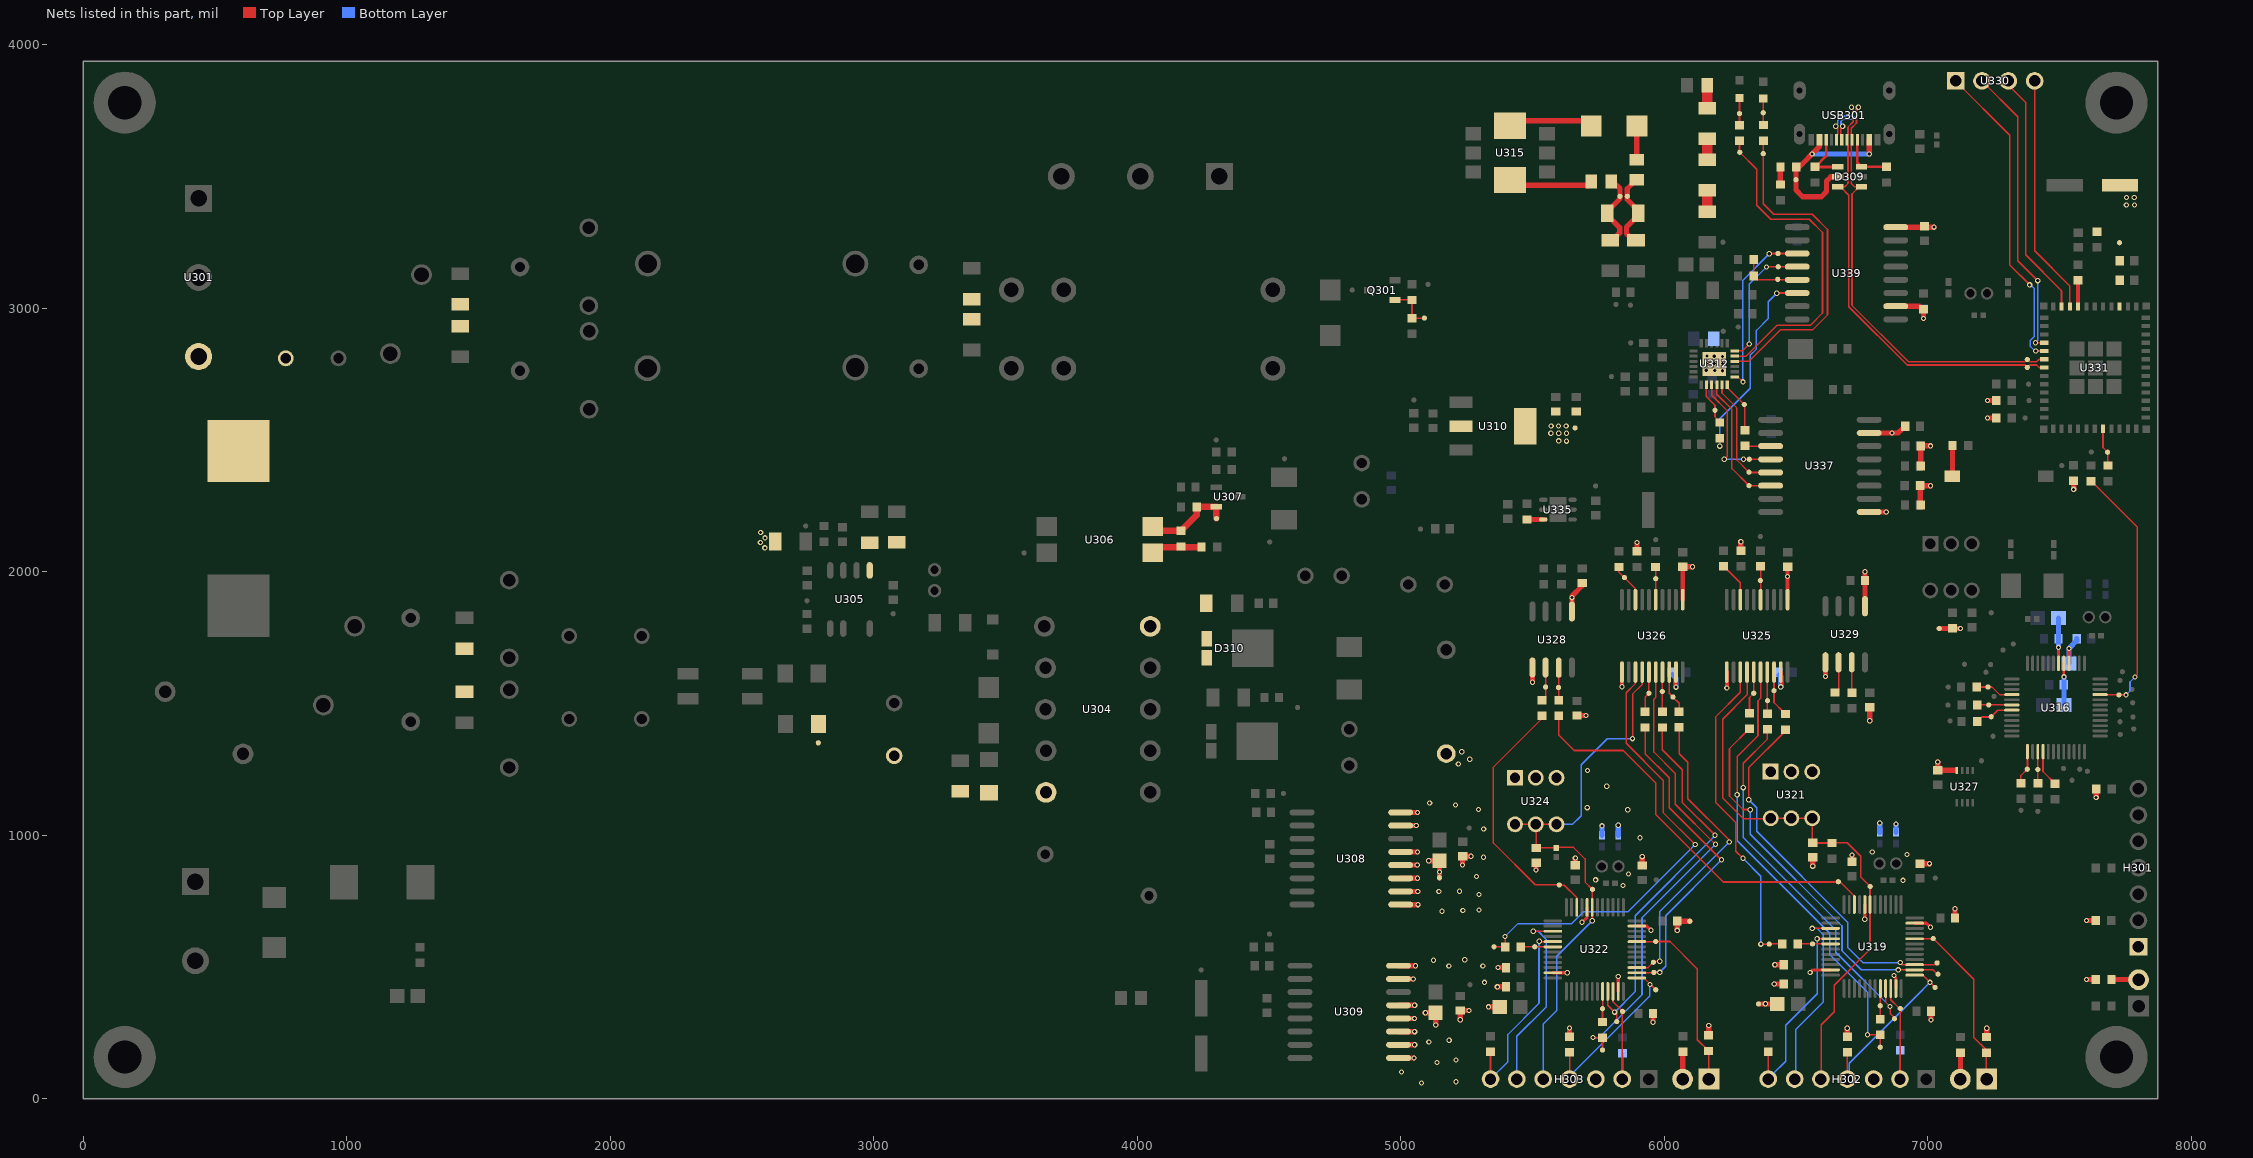
[diagram p0: the nets of this part, all layers, seen from the top]
# Altium PCB MISC84429.PcbDoc (part 4 of 5)
Units mil, origin at the board's own origin, x right, y up, seen from the top; angles counter-clockwise.
Board outline 7874.02 x 3937.01 mil, 4 copper layers (Top Layer, GND, POWER, Bottom Layer); 424 components, 202 nets, 1144 pads, 784 vias.

## Via types
v1: diameter 20, hole 12, Top Layer to Bottom Layer, tented both sides, 695 vias
v2: diameter 20, hole 12, Top Layer to Bottom Layer, 87 vias
v3: diameter 30, hole 15, Top Layer to Bottom Layer, tented both sides, 2 vias

## Nets (pads, with @x,y where several pads share a name; then routed paths per layer and width w, separated by ;. In a path a pad name is that pad's centre, name@x,y a point inside that pad or via, vN(x,y) a via of type N, cw(c..) or ccw(c..) an arc to the next point about the centre after c; other vN are vias at no path point) (continued)
NetD308_1: D308.1 L309.2 | length 97.4
  Top Layer w20: L309.2@5896,3563.04 5896,3659 D308.1@5897,3660
NetD308_2: D308.2 U315.8 | length 299.9
  Top Layer w20: U315.8@5415.01,3691.96 U315.8@5439.06,3716 ; U315.8@5440.06,3711 D308.2@5706,3711
NetD309_3: D309.3 R406.2 USB301.4 | length 203.4
  Top Layer w10: USB301.4@6733.21,3638.49 6733.21,3551.44 6748.98,3535.66 R406.2@6843,3535.66
NetD309_4: D309.4 R408.2 USB301.10 | length 205.2
  Top Layer w10: USB301.10@6615.1,3638.49 6615.1,3577.1 6573.66,3535.66 6573.92,3535.4 D309.4@6658.76,3535.4
NetD309_5: D309.5 R405.2 TP427.1 USB301.2 USB301.11 | length 723
  Top Layer w20: USB301.11@6589.51,3638.49 6589.51,3612.51 6500,3523 TP427.1@6500,3487 6500,3448 6526,3422 6596,3422 6616,3442 6616,3482 6632,3498 D309.5@6658.76,3498 ; v1(6778.49,3584.49) USB301.2@6778.49,3638.49
  Bottom Layer w20: v1(6561.51,3584.49) v1(6778.49,3584.49)
NetD310_1: D310.1 D310.2 R432.1 U304.10
NetF301_1: F301.1 F302.1 U301.3
NetL307_1: L307.1 U312.25
  other v1: 6222,2762 6192,2763 6160,2764 6221,2789 6160,2790 6191,2790 6221,2816 6190,2817 6162,2818
NetL308_2: L308.2 R339.2 | length 70.8
  Top Layer w40: R339.2@6163,3758.22 L308.2@6163,3829
NetL309_1: L309.1 R342.1 R344.2 TP341.1 | length 271.9
  Top Layer w20: R344.2@5877,3263 5857,3283 5857,3307 5901.22,3351.22 R342.1@5901.22,3360 5901.22,3370.78 5860,3412 5860,3453 L309.1@5887,3480
NetL310_1: L310.1 R338.2 R342.2 TP339.1 | length 287.9
  Top Layer w20: R342.2@5793.5,3377.5 5784.78,3368.78 R342.2@5784.78,3360 5784.78,3352.22 5831,3306 5831,3285 R338.2@5808,3262 ; R342.2@5794,3377 5832,3415 5832,3454 L310.1@5805,3481 ; R338.2@5796,3257.22 R338.2@5805.22,3257.22
NetL310_2: L310.2 U315.7 | length 311.6
  Top Layer w20: U315.7@5415.01,3486.04 U315.7@5438.06,3463 ; U315.7@5438.06,3466 L310.2@5710,3466 ; L310.2@5710,3463 L310.2@5715,3468
NetQ301_1: Q301.1 R306.2 R307.1 TP302.1 | length 164.2
  Top Layer w6: Q301.1@4990,3031 5040,3031 5043,3028 R306.2@5043,2961.66 TP302.1@5086.66,2961.66
NetR301_1: R301.1 R304.2
NetR303_1: R303.1 R305.2
NetR308_1: R308.1 R311.2
NetR315_1: R315.1 R316.2 U306.1 | length 157.3
  Top Layer w25: U306.1@4087,2093 R315.1@4244.34,2093
NetR316_1: R316.1 R322.1 TP311.1 U306.2 U307.2 | length 297.9
  Top Layer w25: U306.2@4087.66,2154.66 R316.1@4166,2154.66 4226,2214.66 4226,2242 R322.1@4225,2243 ; R322.1@4236.4,2245.4 U307.2@4300.31,2245.4 TP311.1@4300.31,2203.31
NetR319_2: R319.2 R320.2 U305.5
NetR328_1: R328.1 TP320.1 U312.24 | length 202.5
  Top Layer w6: U312.24@6239.21,2699.79 U312.24@6239.21,2709.33 6239.21,2698.79 6306,2632 R328.1@6306,2544
NetR330_1: R330.1 TP324.1 U312.20 | length 157
  Top Layer w6: U312.20@6160.47,2709.33 6160.47,2663.53 6193,2631 TP324.1@6193,2612 6193,2587 R330.1@6208,2572
NetR334_1: R334.1 TP327.1 U313.2 | length 100.3
  Top Layer w6: R334.1@6376.74,3694.64 U313.2@6376.74,3794.92
NetR334_2: R334.2 TP329.1 U312.4 | length 1279.7
  Top Layer w6: U312.4@6268.4,2797.85 6321.85,2797.85 6441,2917 6563,2917 6620,2974 6620,3298 6562,3356 6416,3356 6376,3396 TP329.1@6376,3586 ; 6376.74,3600.26 6376.74,3609 ; R334.2@6376.74,3635.32 6376.74,3609 ; TP329.1@6378,3588 6376.74,3589.26 6376.74,3609
NetR335_1: R335.1 TP328.1 U314.1 | length 103.8
  Top Layer w6: R335.1@6286,3693.66 TP328.1@6286,3738 U314.1@6286,3797.5
NetR335_2: R335.2 TP330.1 U312.5 | length 1270.2
  Top Layer w6: U312.5@6268.4,2817.53 6310.53,2817.53 6428,2935 6555,2935 6601,2981 6601,3287 6551,3337 6404,3337 6351,3390 6351,3527 6286,3592 R335.2@6286,3634.34
NetR339_1: R339.1 R340.1 | length 65.8
  Top Layer w40: R340.1@6163,3563.22 R339.1@6163,3629
NetR340_2: R340.2 R341.2 | length 75.8
  Top Layer w40: R341.2@6163,3366.22 R340.2@6163,3442
NetR346_2: R346.2 TP346.1 U316.45 | length 999.7
  Top Layer w6: R346.2@7620,2343.34 R346.2@7630.67,2332.67 ; R346.2@7631,2333 7796,2168 7796,1609 v1(7787,1600) ; U316.45@7654.32,1533.21 TP346.1@7724.79,1533.21 ; TP346.1@7726,1532 v1(7753,1532)
  Bottom Layer w6: v1(7753,1532) 7768,1547 7768,1581 v1(7787,1600)
NetR348_1: R348.1 TP366.1 U316.16 | length 145.9
  Top Layer w6: R348.1@7185.66,1562 TP366.1@7229,1562 7244,1562 7272.79,1533.21 U316.16@7319.68,1533.21
NetR349_1: R349.1 TP368.1 U316.18 | length 131.4
  Top Layer w6: R349.1@7188.66,1493 7189.5,1493.84 U316.18@7319.68,1493.84
NetR350_1: R350.1 TP370.1 U316.19 | length 149.9
  Top Layer w6: R350.1@7187.66,1431 7204.66,1448 7240,1448 TP370.1@7241,1449 7266.16,1474.16 U316.19@7319.68,1474.16
NetR351_2: R351.2 U316.28 | length 141.2
  Top Layer w6: U316.28@7437.79,1316.68 7437.79,1240.87 R351.2@7484,1194.66
NetR352_2: R352.2 TP372.1 U316.27 | length 119.9
  Top Layer w6: R352.2@7418.1,1196.76 U316.27@7418.1,1316.68
NetR353_2: R353.2 TP375.1 U316.25 | length 130.3
  Top Layer w6: R353.2@7354,1196.66 7354,1226 TP375.1@7378,1250 7378.73,1250.73 U316.25@7378.73,1316.68
NetR355_1: R355.1 U317.2 | length 90.3
  Top Layer w20: R355.1@7697.66,452 U317.2@7788,452
NetR361_1: R361.1 TP382.1 U319.18 | length 118.7
  Top Layer w6: R361.1@6512.84,586.84 U319.18@6631.55,586.84
NetR362_1: R362.1 U320.2 | length 65
  Top Layer w20: U320.2@7125,109 R362.1@7125,174
NetR364_2: R364.2 TP384.1 U319.32 | length 112
  Top Layer w6: R364.2@6820.53,305.53 U319.32@6820.53,417.55
NetR370_1: R370.1 U323.2 | length 102.1
  Top Layer w20: U323.2@6071,75.22 R370.1@6071,177.34
NetR372_1: R372.1 TP395.1 U322.18 | length 121.7
  Top Layer w6: R372.1@5455.66,576 TP395.1@5509,576 ; TP395.1@5509.16,575.84 U322.18@5577.55,575.84
NetR373_2: R373.2 TP397.1 U322.32 | length 116.1
  Top Layer w6: R373.2@5766,290.66 TP397.1@5766,341 5766.53,341.53 U322.32@5766.53,406.55
NetR378_2: R378.2 TP406.1 U325.18 | length 165.1
  Top Layer w6: U325.18@6416.98,1618.56 6416.98,1503.02 R378.2@6452,1468
NetR379_1: R379.1 TP408.1 U325.5 | length 127.2
  Top Layer w6: R379.1@6365,2020.34 6365.79,2019.55 U325.5@6365.79,1893.44
NetR380_2: R380.2 TP409.1 U325.17 | length 154.2
  Top Layer w6: R380.2@6391.39,1464.39 U325.17@6391.39,1618.56
NetR381_2: R381.2 TP410.1 U325.15 | length 158.2
  Top Layer w6: R381.2@6324,1472 6324,1522 TP410.1@6340,1538 ; R381.2@6328,1467 R381.2@6328,1472 ; TP410.1@6340.2,1538 U325.15@6340.2,1618.56
NetR382_1: R382.1 U325.8 | length 153
  Top Layer w6: R382.1@6226,2020.34 6289.02,1957.32 U325.8@6289.02,1893.44
NetR383_1: R383.1 TP413.1 U326.5 | length 124
  Top Layer w6: U326.5@5967.79,1893.44 5967.79,2017.13 R383.1@5968,2017.34
NetR384_2: R384.2 TP411.1 U326.18 | length 165.6
  Top Layer w6: U326.18@6018.98,1618.56 6018.98,1538.02 TP411.1@6033,1524 6057,1500 R384.2@6057,1468.66
NetR385_2: R385.2 TP414.1 U326.17 | length 151.1
  Top Layer w6: R385.2@5993,1467.66 5993.39,1468.05 U326.17@5993.39,1618.56
NetR386_2: R386.2 TP415.1 U326.15 | length 156.8
  Top Layer w6: R386.2@5928,1467.66 5928,1524 TP415.1@5942,1538 5942.2,1538.2 U326.15@5942.2,1618.56
NetR387_1: R387.1 TP416.1 U326.8 | length 150
  Top Layer w6: R387.1@5828,2017.34 5828,1998 5891.02,1934.98 U326.8@5891.02,1893.44
NetR388_2: R388.2 TP417.1 U328.7 | length 123.8
  Top Layer w6: R388.2@5600,1511.66 U328.7@5600,1635.5
NetR389_2: R389.2 TP418.1 U328.6 | length 109.8
  Top Layer w6: R389.2@5550,1525.66 U328.6@5550,1635.5
NetR393_2: R393.2 U329.7 | length 113.5
  Top Layer w6: R393.2@6712,1542 U329.7@6712,1655.5
NetR395_2: R395.2 U329.6 | length 102.5
  Top Layer w6: R395.2@6662,1553 U329.6@6662,1655.5
NetR401_2: R401.2 U331.8 | length 95.7
  Top Layer w15: U331.8@7571.02,3006.29 R401.2@7571.02,3102.02
NetR403_2: R403.2 TP425.1 U331.31 | length 146.7
  Top Layer w6: U331.31@7665.51,2541.72 7665.51,2470.49 TP425.1@7683,2453 7684,2452 R403.2@7684,2402.66
NetR404_1: R404.1 R405.1 | length 66
  Top Layer w20: R404.1@6441,3468.66 R405.1@6441,3534.66
NetR407_2: R407.2 SW301.1 | length 109.2
  Top Layer w20: SW301.1@7093.83,2362 R407.2@7093.83,2471.17
NetR416_2: R416.2 U335.6 | length 52
  Top Layer w20: R416.2@5489.6,2197.6 U335.6@5541.59,2197.6
PGND: C324.2 C325.1 C328.2 C330.2 C331.1 C369.1 C370.2 C371.2 C372.2 C373.2 C374.2 C375.1 C376.1 C377.2 C378.1 C379.1 C380.2 C381.2 C382.2 C383.2 C384.2 C385.1 C386.1 C387.2 C388.1 C390.2 C392.2 C395.2 C397.2 H302.3 H303.3 R363.2 R368.2 R371.1 R377.2 TP403.1 TP404.1 TP405.1 U308.9 U308.10 U308.11 U308.12 U308.13 U308.15 U308.16 U309.9 U309.10 U309.11 U309.12 U309.13 U309.15 U309.16 U319.8 U319.23 U319.35 U319.47 U321.1 U321.2 U321.3 U322.8 U322.23 U322.35 U322.47 U324.1 U324.2 U324.3 U325.11 U325.19 U326.11 U326.19 U328.5 U329.5 | length 3086.6
  Top Layer w12: U322.23@5577.55,477.42 v1(5632.42,477.42) ; v1(5688,669) 5707.47,688.47 U322.8@5707.47,725.45 ; U322.35@5825.58,406.55 v1(5825.58,463.58) ; U322.47@5896.45,654.58 5934.42,654.58 v1(5950,639) ; v1(6554,478) 6564.42,488.42 U319.23@6631.55,488.42 ; v1(6761.47,680.47) U319.8@6761.47,736.45 ; v1(6872,467) 6871,466 6879.58,457.42 U319.35@6879.58,417.55 ; U319.47@6950.45,665.58 6995.42,665.58 v1(7011,650)
  Top Layer w15: v1(5839.84,1562.84) U326.11@5839.84,1618.56 ; v1(6044.57,1561.43) U326.19@6044.57,1618.56 ; v1(6237.84,1557.84) U325.11@6237.84,1618.56 ; v1(6442.57,1562.43) U325.19@6442.57,1618.56
  Top Layer w20: U309.9@4992.02,154 v1(5051,154) ; U309.10@4992.02,204 v1(5053,204) ; U309.11@4992.02,254 v1(5053,254) ; U309.12@4992.02,304 v1(5052,304) ; U309.13@4992.02,354 v1(5053,354) ; U309.15@4992.02,454 v1@5047,454 ; U309.16@4992.02,504 v1(5056,504) ; U308.9@5000.02,736 v1(5066,736) ; U308.10@5000.02,786 v1(5065,786) ; U308.11@5000.02,836 v1(5064,836) ; U308.12@5000.02,886 v1(5063,886) ; U308.13@5000.02,936 v1(5064,936) ; U308.15@5000.02,1036 v1(5059,1036) ; U308.16@5000.02,1086 v1(5064,1086) ; v1(5093.63,325.63) C331.1@5133,325.63 v1(5133,279) ; v1(5106.63,902.63) C325.1@5147,902.63 v1(5147,860) TP403.1@5147,838 ; v1(5226,299) C330.2@5226,334.44 v1(5259.44,334.44) ; v1(5235,886) C324.2@5235,919.44 v1(5266.56,919.44) ; v1(5333,348) C385.1@5375.63,348 ; v1(5367,424) C386.1@5399.44,424 ; v1(5369,497) C387.2@5399.44,497 ; v1(5500,1580) U328.5@5500,1635.5 ; v1(5514,867) C388.1@5514,895.44 ; R377.2@5641,234.66 v1(5641,268) ; C381.2@5663,885.56 v1(5663,913) ; C395.2@5669,1453.44 v1(5703.44,1453.44) ; C382.2@5917,884.56 v1(5917,918) ; v1(5957.56,289.56) C384.2@5957.56,323 ; v1(6049.56,638.44) C383.2@6049.56,674 ; C383.2@6057,673 TP404.1@6097,673 ; R371.1@6169,239.66 v1(6169,277) ; TP405.1@6358,359 v1@6384,359 ; v1(6384,360) v1@6384,359 ; v1(6418,435) C376.1@6453.44,435 ; v1(6420,508) C377.2@6453.44,508 ; C375.1@6422,359 v1@6384,359 ; v1(6564,882) C378.1@6564,915.44 ; v1(6612,1602) U329.5@6612,1655.5 ; R368.2@6695,234.66 v1(6695,267) ; C371.2@6713,898.56 v1(6713,924) ; v1(6780,1434) C397.2@6780,1485.44 ; C372.2@6971,891.56 v1(7006.56,891.56) ; v1(7012.56,298.56) C374.2@7012.56,331 ; C373.2@7103.56,685 v1(7103.56,720.56) ; R363.2@7224,233.66 v1(7224,267)
  Bottom Layer w20: C379.1@5764,999.46 v1(5764,1035) ; C380.2@5826,999.46 v1(5826,1037) ; C392.2@6032,1609 6044.57,1596.43 v1(6044.57,1561.43) ; C390.2@6436,1607 6442.57,1600.43 v1(6442.57,1562.43) ; C369.1@6818,1010.46 v1(6818,1046) ; C370.2@6880,1010.46 v1(6880,1042)
  other v1: 5079,59 5210,64 5003,101 5138,137 5210,146 5107,215 5184,221 5318,441 5048,454 5183,503 5312,503 5125,525 5243,527 5157,711 5236,714 5297,716 5297,774 5145,786 5223,787 5844,809 6906,828 5740,830 5288,843 5865,852 5314,916 6922,926 6790,936 5908,990 5315,1023 5862,1096 5295,1097 5708,1104 5208,1114 5110,1122 5782,1185 5709,1245
  other v2: 5219,1270 5262,1288 5232,1316
STPM32_CS: TP323.1 U312.21 U337.12 | length 484.1
  Top Layer w6: U312.21@6180.16,2709.33 6180.16,2668.84 6240,2609 6240,2438 v2(6228,2426) ; v2(6301,2426) TP323.1@6323,2426 ; TP323.1@6328,2426 U337.12@6403.98,2426
  Bottom Layer w6: v2(6228,2426) v2(6301,2426)
STPM32_EN: R336.1 R337.2 TP337.1 U339.5 | length 228.2
  Top Layer w6: R337.2@6339.66,3123.34 R336.1@6339.66,3184 ; R337.2@6342,3118 6353,3107 U339.5@6504.98,3107
STPM32_INT1: TP332.1 U312.6 U339.4 | length 473.6
  Top Layer w6: U312.6@6268.4,2837.22 6296.22,2837.22 v2(6323,2864) ; v2(6388,3156) U339.4@6477,3156
  Bottom Layer w6: v2(6323,2864) 6323,3091 v2(6388,3156)
STPM32_MISO: R328.2 U337.11 | length 85
  Top Layer w6: R328.2@6319,2476 U337.11@6403.98,2476
STPM32_MOSI: TP321.1 U312.23 U337.13 | length 445.1
  Top Layer w6: U312.23@6219.52,2709.33 6219.52,2677.48 6276,2621 6276,2423 TP321.1@6318,2381 ; TP321.1@6328,2376 U337.13@6403.98,2376
STPM32_SCK: TP322.1 U312.22 U337.14 | length 509.7
  Top Layer w6: U312.22@6199.84,2709.33 6199.84,2673.16 6257,2616 6257,2426 6257,2391 TP322.1@6319,2329 ; TP322.1@6324,2326 U337.14@6403.98,2326
STPM32_SYN: R330.2 U339.6 | length 771.8
  Top Layer w6: v2(6211,2476) R330.2@6211,2506.34 ; v2@6433,3057 U339.6@6504.98,3057
  Bottom Layer w6: v2(6211,2476) 6211,2580 6327,2696 6327,2822 6350,2845 6350,2915 6395,2960 6395,3024 v2(6427,3056)
STPM32_ZCR: TP325.1 U312.1 U339.3 | length 645.2
  Top Layer w6: U312.1@6268.42,2738.79 6280.21,2738.79 v2(6299,2720) ; v2(6399,3206) 6400,3207 TP325.1@6432,3207 U339.3@6478,3207
  Bottom Layer w6: v2(6299,2720) 6299,3106 v2(6399,3206)
TCK: U330.2 U331.15 | length 1116.6
  Top Layer w6: U330.2@7206,3862 7342,3726 7342,3180 7416,3106 v1@7419,3106 ; v1(7409.49,2868.49) U331.15@7442.09,2868.49
  Bottom Layer w6: v1(7409.49,2868.49) 7418,2877 v1@7418,3103
  other v1: 7418,3104
TDI: U330.3 U331.10 | length 924.8
  Top Layer w6: U330.3@7305,3847 7372,3780 7372,3202 7508.03,3065.97 U331.10@7508.03,3006.29
TDO: U330.1 U331.16 | length 1196.1
  Top Layer w6: U330.1@7106,3862 7312,3656 7312,3163 v1(7387,3088) v1@7388,3087 ; v1(7410,2837) U331.16@7442.09,2837
  Bottom Layer w6: v1@7387,3087 v1(7387,3088) ; v1@7391,3087 7405,3073 7405,2893 7390,2878 7390,2854 v1@7405,2839 ; v1@7406.5,2840.5 v1(7410,2837)
TMS: U330.4 U331.9 | length 912
  Top Layer w6: U330.4@7406,3863 U330.4@7406,3862 7406,3217 7539.53,3083.47 U331.9@7539.53,3006.29
U575_BOOT0: R363.1 TP380.1 U319.44 U320.1 | length 646.3
  Top Layer w6: U319.44@6950.45,606.53 TP380.1@7014.53,606.53 ; TP380.1@7021,607 7175,453 7175,232 7222,185 U320.1@7222,108
U575_BOOT0_2: R371.2 TP393.1 U322.44 U323.1 | length 706.8
  Top Layer w6: U322.44@5896.45,595.53 TP393.1@5967.53,595.53 ; TP393.1@5968,596 6022,596 6126,492 6126,223.34 R371.2@6169,180.34 U323.1@6169,75.2
U575_IWDG1_OUT_PB0: R361.2 TP381.1 U325.13 | length 1219.7
  Top Layer w6: U325.13@6289.02,1618.56 6289.02,1542.02 6195,1448 6195,1125 6272,1048 6272,939 v1(6299,912) ; v1(6367,586) TP381.1@6399,586 ; TP381.1@6402,587 R361.2@6448.34,587
  Bottom Layer w6: v1@6300,911 6367,844 v1(6367,586)
U575_IWDG2_OUT_PB0: R372.2 TP394.1 U326.13 | length 1725.3
  Top Layer w6: TP394.1@5354,576 R372.2@5396.34,576 v1(5396.34,615.34) ; U326.13@5891.02,1618.56 5891.02,1575.02 5856,1540 5856,1348 5996,1208 5996,1086 v1(6118,964)
  Bottom Layer w6: v1(5396.34,615.34) 5445,664 5649,664 5694,709 5863,709 v1(6118,964)
U575_NRST: C378.2 H302.5 R365.1 TP378.1 U319.7 U321.4 U321.5 U321.6 U325.14 | length 2104.1
  Top Layer w6: U325.14@6314.61,1618.56 6314.61,1532.61 6222,1440 6222,1141 6301,1062 U321.4@6396,1062 ; U321.4@6415,1065 6416.46,1063.54 U321.5@6482.85,1063.54 U321.6@6561.59,1063.54 6561.59,972.41 C378.2@6566,968 ; U321.6@6560,1052 U321.6@6566.21,1045.79 ; C378.2@6566.21,970.56 6566.21,969.79 R365.1@6630,969.79 ; H302.5@6596,107 6596,280 6645,329 6645,430.26 6781.16,566.42 U319.7@6781.16,736.45 TP378.1@6781.16,805.84 ; 6609,971 6695,971 6746,920 6746,841 TP378.1@6781.16,805.84 ; TP378.1@6782,805 TP378.1@6781.16,805.84
U575_NRST_2: C388.2 H303.5 R374.1 TP391.1 U322.7 U324.4 U324.5 U324.6 U326.14 | length 2165.1
  Top Layer w6: U324.4@5434.11,1040.54 U324.5@5512.85,1040.54 ; U324.5@5510,1022 5514,1018 C388.2@5514,952.56 ; C388.2@5512.91,952.56 C388.2@5514,952.56 ; U324.5@5512.91,1040.47 U324.5@5512.85,1040.54 ; C388.2@5514,950.56 C388.2@5514,952.56 ; U324.6@5591.59,1040.54 U324.5@5512.85,1040.54 ; R374.1@5593,952.56 C388.2@5514,952.56 ; R374.1@5593,953 5656,953 5700,909 5700,822 TP391.1@5727.16,794.84 ; v1(5727.16,674.84) U322.7@5727.16,725.45 TP391.1@5727.16,794.84 ; TP391.1@5728,794 TP391.1@5727.16,794.84 ; v1(5880,1366) 5880,1535 5916.61,1571.61 U326.14@5916.61,1618.56
  Bottom Layer w6: H303.5@5541,74 5541,238 5541,283 5565.5,307.5 5592,334 5592,539.68 v1(5727.16,674.84) ; U324.6@5591.59,1040.54 5652.54,1040.54 5685,1073 5685,1267 5784,1366 v1(5880,1366)
U575_PA0_1: R388.1 TP379.1 U319.10 | length 1549.7
  Top Layer w6: R388.1@5600,1452.34 5600,1380 5659,1321 5845,1321 5968,1198 5968,1078 6224,822 6656,822 6668,822 6722.1,767.9 U319.10@6722.1,736.45
U575_PA0_2: R389.1 TP392.1 U322.10 | length 997.5
  Top Layer w6: R389.1@5536,1452.34 5536,1442 5352,1258 5352,970 5511,811 TP392.1@5602,811 ; TP392.1@5602,810 5621,810 5668.1,762.9 U322.10@5668.1,725.45
U575_PA13_SWDIO: H302.2 R366.1 TP387.1 U319.34 | length 432.8
  Top Layer w6: U319.34@6859.9,417.55 6859.9,375.1 TP387.1@6891,344 ; H302.2@6896,84 TP387.1@6896,342
  Bottom Layer w6: H302.2@6896,95 R366.1@6896,183.34
U575_PA13_SWDIO_2: H303.2 R375.1 TP400.1 U322.34 | length 427.4
  Top Layer w6: U322.34@5805.9,406.55 5805.9,367.1 5841,332 H303.2@5841,74
  Bottom Layer w6: H303.2@5842,92 R375.1@5842,172.34
U575_PA14_SWCLK: H302.4 R368.1 TP388.1 U319.37 | length 637.6
  Top Layer w6: H302.4@6695,103 R368.1@6695,186.34 ; U319.37@6950.45,468.73 6981.27,468.73 v1(7009,441) TP388.1@7026,424
  Bottom Layer w6: 6702,108 6702,134 6954.5,386.5 v1(7009,441)
U575_PA14_SWCLK_2: H303.4 R377.1 TP401.1 U322.37 | length 676.8
  Top Layer w6: H303.4@5641,74 R377.1@5641,175.34 ; U322.37@5896.45,457.73 5923.27,457.73 TP401.1@5968,413
  Bottom Layer w6: H303.4@5641,74 5641,85 5946,390 v1(5946,433)
U575_SPI1_A11_MISO1: R364.1 TP386.1 U325.16 | length 1708.2
  Top Layer w6: v1@6276,1154 v1(6277,1153) v1@6278.5,1151.5 ; v1@6277,1155 6277,1298 6356,1377 6356,1509 6365.79,1518.79 U325.16@6365.79,1618.56 ; v1(6771.66,242.34) R364.1@6820,242.34 TP386.1@6820,201
  Bottom Layer w6: v1(6277,1153) 6277,978 6628,627 6628,547 6772,403 v1@6772,245 ; v1@6770.5,243.5 v1(6771.66,242.34)
U575_SPI1_PA11_MISO2: R373.1 TP399.1 U326.16 | length 1776.2
  Top Layer w6: v1(5730.34,231.34) R373.1@5766,231.34 TP399.1@5766,184 ; U326.16@5967.79,1618.56 5967.79,1521.79 5961,1515 5961,1315 6042,1234 6042,1117 v1@6194.5,964.5
  Bottom Layer w6: v1(5730.34,231.34) 5753.34,231.34 5916,394 5916,686 v1(6195,965)
U575_SPI1_PA12_MOSI: R380.1 TP385.1 U319.33 | length 1439.6
  Top Layer w6: v1@6300,1184 6300,1273 6392,1365 R380.1@6392,1401.34 ; U319.33@6840.21,417.55 6840.21,366.79 v1@6857.5,349.5 ; v1@6858,349 6858,323 TP385.1@6873,308
  Bottom Layer w6: v1(6300,1180) 6300,991 6651,640 6651,555 v1(6857,349)
U575_SPI1_PA12_MOSI_2: R385.1 TP398.1 U322.33 | length 1452.1
  Top Layer w6: U322.33@5786.21,406.55 5786.21,353.79 v1(5812,328) 5820,320 TP398.1@5820,292 ; R385.1@5993,1408.34 5993,1324 6069,1248 6069,1124 6192,1001 v1@6197,1001
  Bottom Layer w6: v1(5812,328) 5890,406 5890,694 6193,997 v1(6193,999)
U575_SPI1_PA15_NSS1: R381.1 TP389.1 U319.38 | length 1467.4
  Top Layer w6: v1@6322,1096 v1(6327,1096) ; v1@6322,1097 6299,1097 6248,1148 6248,1328.34 R381.1@6323,1403.34 ; v1(6888.42,488.42) U319.38@6950.45,488.42 7020.58,488.42 TP389.1@7039,470
  Bottom Layer w6: v1(6327,1096) 6327,1003 6675,655 6675,561 6747.58,488.42 v1(6888.42,488.42)
U575_SPI1_PA15_NSS2: R386.1 TP402.1 U322.38 | length 1233.9
  Top Layer w6: U322.38@5896.45,477.42 TP402.1@5961,477.42 ; R386.1@5928,1408.34 5928,1308 6019,1217 6019,1104 6217,906 v1(6218,906) ; TP402.1@5961,479 v1(5983,479)
  Bottom Layer w6: v1(5983,479) 6006,502 6006,694 v1(6218,906)
U575_SPI1_PB3_SCK: R378.1 TP383.1 U319.39 | length 1405.8
  Top Layer w6: v1@6321,1138 6321,1256 6461,1396 R378.1@6461,1400.34 ; v1(6896,516) 6903.9,508.1 U319.39@6950.45,508.1 7029.1,508.1 TP383.1@7036,515
  Bottom Layer w6: v1(6321,1134) 6351,1104 6351,1014 6697,668 6697,573 6754,516 v1(6896,516)
U575_SPI1_PB3_SCK_2: R384.1 TP396.1 U322.39 | length 1165.8
  Top Layer w6: U322.39@5896.45,497.1 5939.1,497.1 TP396.1@5959,517 5963,521 v1(5983,521) ; R384.1@6057,1409.34 6057,1309 6090,1276 6090,1138 v1@6247,981
  Bottom Layer w6: v1(5983,521) 5983,710 v1(6247,974)
U575_USART3_RX: H302.6 U319.15 | length 688.3
  Top Layer w6: v1(6561.9,645.9) U319.15@6631.55,645.9
  Bottom Layer w6: H302.6@6499,98 6499,206 6499,262 6603,366 6603,623 6580.1,645.9 v1(6561.9,645.9)
U575_USART3_RX_2: H303.6 U322.15 | length 712.7
  Top Layer w6: v1(5503.1,634.9) U322.15@5577.55,634.9
  Bottom Layer w6: H303.6@5441,74 5441,236 5552,347 5552,605 5522.1,634.9 v1(5503.1,634.9)
U575_USART3_TX: H302.7 R367.1 U319.17 | length 730.1
  Top Layer w6: H302.7@6395,94 R367.1@6395,188.34 ; v1(6580.47,606.53) U319.17@6631.55,606.53
  Bottom Layer w6: H302.7@6411,92 6461,142 6461,278 6580.47,397.47 v1(6580.47,606.53)
U575_USART3_TX_2: H303.7 R376.1 U322.17 | length 758.8
  Top Layer w6: H303.7@5341,74 R376.1@5341,177.34 ; v1(5526,597) 5525.94,597 5524.47,595.53 U322.17@5577.55,595.53
  Bottom Layer w6: H303.7@5341,74 5407,140 5407,243.34 5525,361.34 5525,597 v1(5526,597)
USB_D+: D309.6 TP421.1 U331.18 USB301.6 USB301.8 | length 1828.7
  Top Layer w6: USB301.8@6654.47,3638.49 6654.47,3655.47 6658.31,3659.31 v1@6658.31,3683 ; D309.6@6658.76,3460.6 D309.6@6671,3460.6 ; v1(6711,3762) 6718,3755 6718,3707.29 6697.69,3686.97 6697.69,3659.69 6693.85,3655.85 USB301.6@6693.85,3638.49 6693.85,3621.15 6697.69,3617.31 6697.69,3473 6685.28,3460.6 D309.6@6671,3460.6 ; U331.18@7442.09,2774.01 7423,2774.01 7413.26,2783.75 7386.75,2783.75 TP421.1@7378,2775 7369.25,2783.75 6922.28,2783.75 6701,3005.03 6701,3428 6671,3458 D309.6@6671,3460.6
  Bottom Layer w6: v1(6651.31,3690) 6651.31,3690.87 6659,3698.56 6659,3713 6675,3729 6710,3729 6718,3737 6718,3755 v1(6711,3762)
USB_D-: D309.1 TP420.1 U331.17 USB301.5 USB301.7 | length 1808.3
  Top Layer w6: v1@6670.31,3683 6670.31,3658.69 6674.15,3654.85 USB301.7@6674.15,3638.49 ; v1(6737,3762) 6730,3755 6730,3702.31 6709.69,3682 6709.69,3658.31 6713.53,3654.47 USB301.5@6713.53,3638.49 6713.53,3618.53 6709.69,3614.69 6709.69,3473 6722.08,3460.6 D309.1@6740.6,3460.6 ; D309.1@6749.24,3460.6 D309.1@6740.6,3460.6 ; U331.17@7442.09,2805.5 7423,2805.5 7413.26,2795.75 7387.25,2795.75 TP420.1@7378,2805 7368.75,2795.75 6927.25,2795.75 6713,3010 6713,3433 D309.1@6740.6,3460.6
  Bottom Layer w6: v1(6677.31,3690) 6671,3696.31 6671,3708.03 6679.97,3717 6714.97,3717 6730,3732.03 6730,3755 v1(6737,3762)
VBUS: C312.1 C313.2 L303.2 R313.2 R317.1 TP307.1 U304.5
  other v1: 2587,2090 2570,2110 2588,2128 2571,2148
VCC_3V3: C334.2 C335.1 C363.1 C364.1 C365.1 C366.2 C367.2 C368.2 C389.1 C391.1 C393.1 C394.1 C396.1 C398.1 C399.2 C400.1 C417.1 C419.1 H301.1 R326.1 R327.1 R329.1 R331.1 R332.1 R354.2 R355.2 R357.2 R358.2 R390.1 R391.1 R396.2 R397.2 R398.2 R400.2 TP319.1 TP345.1 TP419.1 U310.2 U310.4 U316.4 U316.5 U316.6 U325.1 U326.1 U327.8 U328.1 U329.1 U331.3 U337.1 U337.7 U339.10 U339.16 | length 2155.5
  Top Layer w11: U316.6@7496.84,1651.32 v1@7496.84,1711.16 ; v1@7516.53,1607.53 U316.5@7516.53,1651.32 ; U316.4@7536.21,1651.32 v1(7536.21,1708.21)
  Top Layer w16: U326.1@6070.16,1893.44 C391.1@6070.16,2009.16 ; U325.1@6468.16,1893.44 v1@6468.16,1983 ; v1(6468.16,1981.16) v1@6468.16,1983 ; C389.1@6468.16,2005.16 v1@6468.16,1983
  Top Layer w20: U328.1@5650,1848.5 v1(5650,1901) ; v1@5650,1900 5650,1907 5689,1946 C394.1@5689,1956.44 ; R391.1@5897,2076.66 v1(5897,2110) ; C391.1@6070,2018.44 v1(6107.56,2018.44) ; R390.1@6291,2079.66 v1(6291,2113) ; U329.1@6762,1868.5 C396.1@6762,1968 ; C396.1@6762.56,1966 v1(6762.56,1999.56) ; U337.1@6778.02,2226 v2(6843,2226) ; U337.7@6778.02,2526 v2@6863,2526 ; v2(6865,2526) v2@6863,2526 ; U339.10@6879.02,3007 6968,3007 R331.1@6976,2999 ; U339.16@6879.02,3307 v2(7024,3307) ; C417.1@6908,2546 6888,2526 v2@6863,2526 ; R329.1@6972.32,2256.68 R327.1@6972.32,2325.75 v2(7010.75,2325.75) ; R332.1@6973.32,2401 R326.1@6973.32,2471.32 ; R326.1@6974.32,2477.1 v2(7011.1,2477.1) ; v2(6983.89,2960.11) R331.1@6983.89,2995.89 ; v1(7038,1277) C393.1@7038,1245.56 7105,1245.56 ; TP345.1@7044,1784 v1(7124,1784) ; v1(7227,2583) R397.2@7260.34,2583 ; v1(7227,2649) R396.2@7260.34,2649 ; v1(7554,2312) R398.2@7554,2344.34 ; v1(7603,452) R355.2@7638.34,452 ; v1(7603,676) R357.2@7637.34,676 ; v1(7639.34,1142.34) R358.2@7639.34,1175
  Bottom Layer w20: v1(7496.37,1712.37) C366.2@7496.37,1824 ; C368.2@7517.37,1493 v1(7517.37,1600.37) ; v1(7536.21,1708.21) 7536.21,1651.16 C367.2@7536.37,1651 ; v1@7538,1710 7565.44,1737.44 C364.1@7565.44,1745
  other v1: 5629,2495 5600,2496 5570,2525 5600,2525 5629,2525 5571,2552 5599,2552 5628,2552 7754,3391 7785,3391 7755,3420 7784,3420